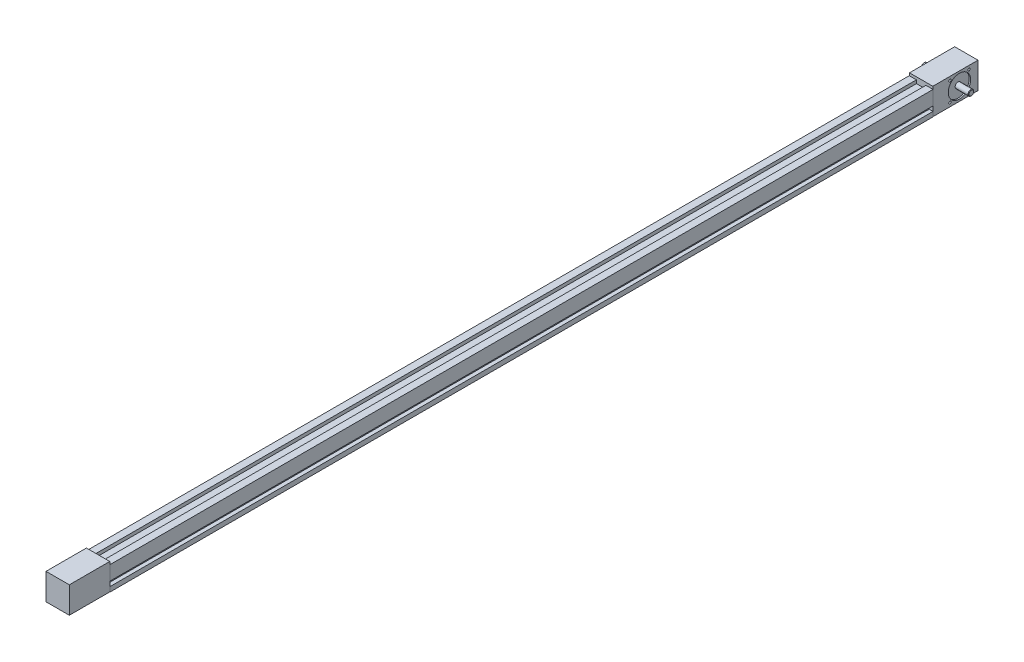
from build123d import *

# Parameters (mm, degrees)
EXTRUDE_671_DEPTH        = 1730
SKETCH_2_W               = 49
SKETCH_2_H               = 55.5
EXTRUDE_1_DEPTH          = 85
SKETCH_4_W               = 49
SKETCH_4_H               = 55.5
EXTRUDE_3_DEPTH          = 95
SKETCH_9_R               = 23.5
CUT_EXTRUDE_5_DEPTH      = 3
SKETCH_10_R              = 6
EXTRUDE_4_DEPTH          = 28
CHAMFER_1_SIZE           = 1
PATTERN_CIRCULAR_1_COUNT = 4


with BuildPart() as part:
    # 草图1 → Extrude 671 (new body)
    with BuildSketch(Plane.XY):
        Polygon((15, 50), (15, 43), (35, 43), (35, 50), (50, 50), (50, 20), (42, 20), (42, 10), (50, 10), (50, 0), (0, 0), (0, 10), (8, 10), (8, 20), (0, 20), (0, 50), align=None)
    extrude(amount=EXTRUDE_671_DEPTH)

    # 草图2 → 凸台-拉伸1 (add)
    with BuildSketch(Plane.XY.offset(1730)):
        with Locations((25, 27.75)):
            Rectangle(SKETCH_2_W, SKETCH_2_H)
    extrude(amount=EXTRUDE_1_DEPTH)

    # 草图4 → 凸台-拉伸3 (add)
    with BuildSketch(Plane(origin=(0, 0, 0), x_dir=(-1, 0, 0), z_dir=(0, 0, -1))):
        with Locations((-25, 27.75)):
            Rectangle(SKETCH_4_W, SKETCH_4_H)
    extrude(amount=EXTRUDE_3_DEPTH)

    # 草图9 → 切除-拉伸5 (cut)
    with BuildSketch(Plane(origin=(49.5, 0, 0), x_dir=(0, 0, -1), z_dir=(1, 0, 0))):
        with Locations((56, 27.75)):
            Circle(SKETCH_9_R)
    cut_extrude_5 = extrude(amount=-CUT_EXTRUDE_5_DEPTH, mode=Mode.SUBTRACT)

    # 草图10 → 凸台-拉伸4 (add)
    with BuildSketch(Plane(origin=(46.5, 0, 0), x_dir=(0, 0, -1), z_dir=(1, 0, 0))):
        with Locations((56, 27.75)):
            Circle(SKETCH_10_R)
    extrude_4 = extrude(amount=EXTRUDE_4_DEPTH)

    # 倒角1
    chamfer_1_edges = [part.edges().sort_by_distance(p)[0] for p in [
        (74.5, 27.75, -50),
    ]]
    chamfer(chamfer_1_edges, length=CHAMFER_1_SIZE)

    # 草图12 → M5 螺纹孔1 (revolve, cut)
    with BuildSketch(Plane(origin=(50, 47.75, -76), x_dir=(0, 0, -1), z_dir=(0, 1, 0))):
        Polygon((0, 0), (0, 15.2618073), (2.1, 14), (2.1, 10), (2.5, 10), (2.5, 0), align=None)
    hole_wizard_m5_1 = revolve(axis=Axis((56.35, 47.75, -76), (-1, 0, 0)), mode=Mode.SUBTRACT)

    # 阵列(圆周)1: M5 螺纹孔1 ×4 about axis
    pattern_circular_1_axis = Axis((0, 27.75, -56), (1, 0, 0))
    for i in range(1, PATTERN_CIRCULAR_1_COUNT):
        add(hole_wizard_m5_1.rotate(pattern_circular_1_axis, i * 360 / PATTERN_CIRCULAR_1_COUNT), mode=Mode.SUBTRACT)

    # 镜向1: 切除-拉伸5, 凸台-拉伸4, M5 螺纹孔1 across plane
    add(cut_extrude_5.mirror(Plane(origin=(25, 0, 0), x_dir=(0, 0, 1), z_dir=(1, 0, 0))), mode=Mode.SUBTRACT)
    add(extrude_4.mirror(Plane(origin=(25, 0, 0), x_dir=(0, 0, 1), z_dir=(1, 0, 0))))
    add(hole_wizard_m5_1.mirror(Plane(origin=(25, 0, 0), x_dir=(0, 0, 1), z_dir=(1, 0, 0))), mode=Mode.SUBTRACT)

    # 镜向1 copy 1 sketch → 镜向1 copy 1 (revolve, cut)
    with BuildSketch(Plane(origin=(0, 47.75, -36), x_dir=(0, 1, 0), z_dir=(0, 0, 1))):
        Polygon((0, 0), (0, -15.2618073), (2.1, -14), (2.1, -10), (2.5, -10), (2.5, 0), align=None)
    revolve(axis=Axis((-6.35, 47.75, -36), (-1, 0, 0)), mode=Mode.SUBTRACT)

    # 镜向1 copy 2 sketch → 镜向1 copy 2 (revolve, cut)
    with BuildSketch(Plane(origin=(0, 7.75, -36), x_dir=(0, 0, 1), z_dir=(0, -1, 0))):
        Polygon((0, 0), (0, -15.2618073), (2.1, -14), (2.1, -10), (2.5, -10), (2.5, 0), align=None)
    revolve(axis=Axis((-6.35, 7.75, -36), (-1, 0, 0)), mode=Mode.SUBTRACT)

    # 镜向1 copy 3 sketch → 镜向1 copy 3 (revolve, cut)
    with BuildSketch(Plane(origin=(0, 7.75, -76), x_dir=(0, -1, 0), z_dir=(0, 0, -1))):
        Polygon((0, 0), (0, -15.2618073), (2.1, -14), (2.1, -10), (2.5, -10), (2.5, 0), align=None)
    revolve(axis=Axis((-6.35, 7.75, -76), (-1, 0, 0)), mode=Mode.SUBTRACT)


solid = part.part
